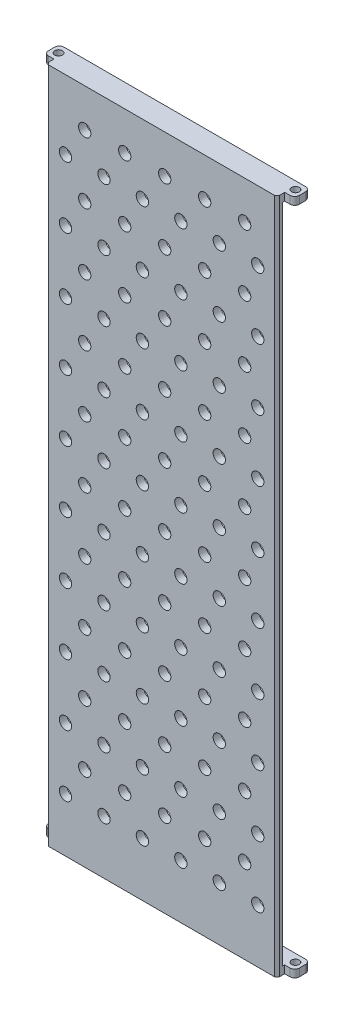
SolidWorks part; units mm, degrees
ref_plane "Front Plane" through (0, 0, 0) normal (0, 0, 1) x (1, 0, 0)
ref_plane "Top Plane" through (0, 0, 0) normal (0, 1, 0) x (1, 0, 0)
ref_plane "Right Plane" through (0, 0, 0) normal (1, 0, 0) x (0, 0, -1)
other "Configuration Table"
sketch "Sketch1" plane through (0, 0, 0) normal (0, 0, 1) x (1, 0, 0)
  line L1 (0, 0) -> (150, 0)
  line L2 (0, 0) -> (0, 430)
  line L3 (0, 430) -> (150, 430)
  line L4 (150, 0) -> (150, 430)
  dimension "D1" = 430
  dimension "D2" = 150
extrude "Boss-Extrude1" add sketch "Sketch1" along normal blind 5
sketch "Sketch2" plane through (0, 0, 5) normal (0, 0, 1) x (1, 0, 0)
  line L0 (0, 410) -> (150, 410) construction
  line L1 (0, 430) -> (0, 0) construction
  line L2 (150, 0) -> (150, 430) construction
  line L3 (0, 390) -> (150, 390) construction
  line L4 (150, 430) -> (0, 430) construction
  line L5 (25, 430) -> (25, 390) construction
  line L6 (12.5, 430) -> (12.5, 390) construction
  circle A0 centre (25, 410) radius 4
  circle A1 centre (51, 410) radius 4
  circle A2 centre (77, 410) radius 4
  circle A3 centre (103, 410) radius 4
  circle A4 centre (129, 410) radius 4
  circle A5 centre (12.5, 390) radius 4
  circle A6 centre (37.5, 390) radius 4
  circle A7 centre (62.5, 390) radius 4
  circle A8 centre (87.5, 390) radius 4
  circle A9 centre (112.5, 390) radius 4
  circle A10 centre (137.5, 390) radius 4
  dimension "D3" = 8
  dimension "D7" = 8
  dimension "D1" = 20
  dimension "D2" = 20
  dimension "D4" = 25
  dimension "D6" = 12.5
  dimension "D5" = 5
  dimension "D8" = 6
extrude "Cut-Extrude1" cut sketch "Sketch2" against normal up to next
pattern_linear "LPattern1" count 10 spacing 40 along (0, -1, 0) of "Cut-Extrude1"
sketch "Sketch3" plane through (0, 0, 0) normal (0, -1, 0) x (-1, 0, 0)
  line L0 (0, -5) -> (-150, -5) construction
  line L1 (6.5, 10) -> (-156.5, 10)
  line L2 (6.5, 10) -> (6.5, -5)
  line L3 (6.5, -5) -> (-156.5, -5)
  line L4 (-156.5, 10) -> (-156.5, -5)
  line L5 (0, -5) -> (0, 0) construction
  dimension "D1" = 15
  dimension "D2" = 163
  dimension "D3" = 0
  dimension "D4" = 6.5
extrude "Boss-Extrude2" add sketch "Sketch3" along normal blind 5
sketch "Sketch4" plane through (0, 430, 0) normal (0, 1, 0) x (1, 0, 0)
  line L5 (-6.5, 10) -> (156.5, 10)
  line L6 (-6.5, 10) -> (-6.5, -5)
  line L7 (-6.5, -5) -> (156.5, -5)
  line L8 (156.5, 10) -> (156.5, -5)
extrude "Boss-Extrude3" add sketch "Sketch4" along normal blind 5
sketch "Sketch6" plane through (0, 435, 0) normal (0, 1, 0) x (1, 0, 0)
  line L0 (156.5, -5) -> (156.5, 10) construction
  line L1 (-6.5, 10) -> (-6.5, -5) construction
  line L2 (156.5, 10) -> (-6.5, 10) construction
  line L4 (156.5, -5) -> (150, -5)
  line L5 (156.5, -5) -> (156.5, 0)
  line L6 (156.5, 0) -> (150, 0)
  line L7 (150, -5) -> (150, 0)
  line L8 (-6.5, -5) -> (0, -5)
  line L9 (-6.5, -5) -> (-6.5, 0)
  line L10 (-6.5, 0) -> (0, 0)
  line L11 (0, -5) -> (0, 0)
  circle A0 centre (-2, 5) radius 2.5
  circle A1 centre (152, 5) radius 2.5
  dimension "D1" = 4.5
  dimension "D2" = 5
  dimension "D3" = 5
  dimension "D4" = 4.5
  dimension "D5" = 5
  dimension "D6" = 5
  dimension "D7" = 6.5
  dimension "D8" = 5
extrude "Cut-Extrude2" cut sketch "Sketch6" against normal through all both and the other way through all
fillet "Fillet1" radius 3 8 edges at (-6.5, -2.5, -10) (-6.5, 432.5, -10) (156.5, 432.5, -10) (156.5, -2.5, -10) (156.5, -2.5, 0) (-6.5, -2.5, 0) (-6.5, 432.5, 0) (156.5, 432.5, 0)
chamfer "Chamfer1" distance 1.5 angle 45 4 edges at (0, 215, 5) (0, 215, 0) (150, 215, 5) (150, 215, 0)
